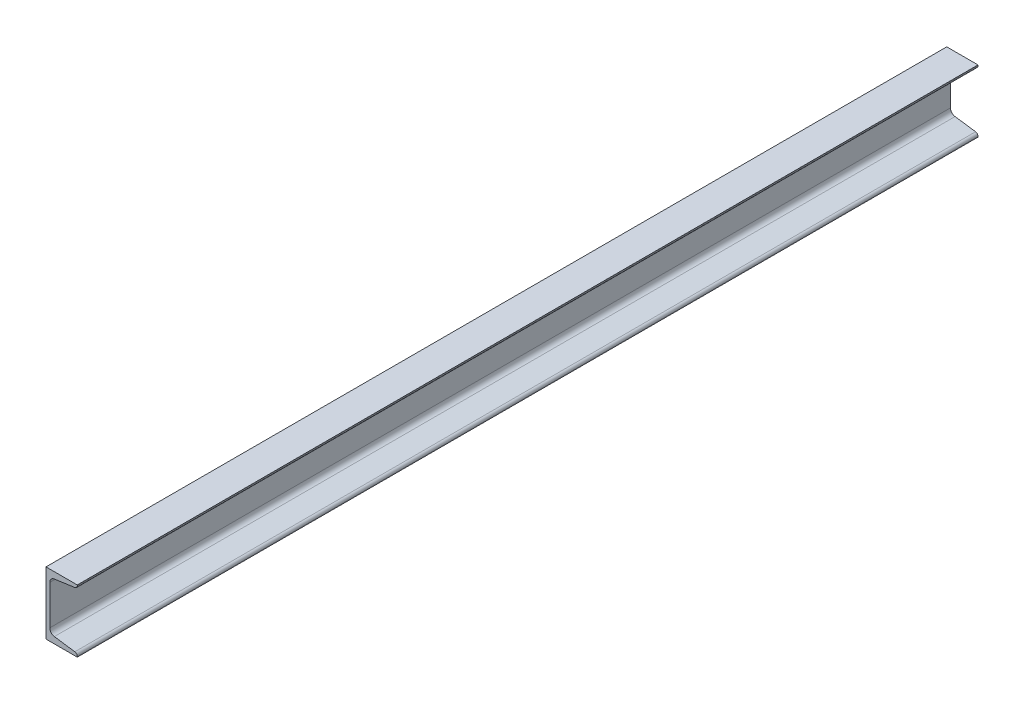
SolidWorks part; units mm, degrees
material "1023 Carbon Steel Plate (SS)"
ref_plane "Front Plane" through (0, 0, 0) normal (0, 0, 1) x (1, 0, 0)
ref_plane "Top Plane" through (0, 0, 0) normal (0, 1, 0) x (1, 0, 0)
ref_plane "Right Plane" through (0, 0, 0) normal (1, 0, 0) x (0, 0, -1)
sketch "Sketch1" plane through (0, 0, 0) normal (0, 0, 1) x (1, 0, 0)
  line L0 (0, 0) -> (-50, 0)
  line L1 (-50, 0) -> (-50, -100)
  line L2 (-50, -100) -> (0, -100)
  line L3 (0, -100) -> (0, -98.9253)
  line L4 (-3.8737, -94.4691) -> (-36.683, -89.8581)
  line L5 (-44, -81.4408) -> (-44, -18.5592)
  line L6 (-36.683, -10.1419) -> (-3.8737, -5.5309)
  line L7 (0, -1.0747) -> (0, 0)
  line L8 (-25, -91.5) -> (-25, -100)
  arc A0 (-36.683, -89.8581) -> (-44, -81.4408) centre (-35.5, -81.4408) cw
  arc A1 (-44, -18.5592) -> (-36.683, -10.1419) centre (-35.5, -18.5592) cw
  arc A2 (0, -98.9253) -> (-3.8737, -94.4691) centre (-4.5, -98.9253) ccw
  arc A3 (-3.8737, -5.5309) -> (0, -1.0747) centre (-4.5, -1.0747) ccw
  dimension "D8" = 8.5
  dimension "D9" = 4.5
  dimension "D1" = 100
  dimension "D2" = 50
  dimension "D3" = 6
  dimension "D4" = 25
  dimension "D5" = 8
  dimension "D6" = 8.5
  dimension "D7" = 8
extrude "Boss-Extrude1" add sketch "Sketch1" along normal blind 1440 contours A3 L6 A1 L5 A0 L4 A2 L3 L2 L1 L0 L7
sketch "Sketch2" plane through (-50, 0, 0) normal (-1, 0, 0) x (0, 0, 1)
  line L0 (0, 0) -> (0, -100) construction
  line L1 (1440, 0) -> (0, 0) construction
  circle A0 centre (73.2, -38) radius 8.5
  circle A1 centre (234.9, -38) radius 8.5
  circle A2 centre (396.6, -38) radius 8.5
  circle A3 centre (558.3, -38) radius 8.5
  circle A4 centre (720, -38) radius 8.5
  circle A5 centre (881.7, -38) radius 8.5
  circle A6 centre (1043.4, -38) radius 8.5
  circle A7 centre (1205.1, -38) radius 8.5
  circle A8 centre (1366.8, -38) radius 8.5
  dimension "D3" = 17
  dimension "D1" = 73.2
  dimension "D2" = 38
  dimension "D4" = 9
extrude "Cut-Extrude1" cut sketch "Sketch2" against normal blind 1440
